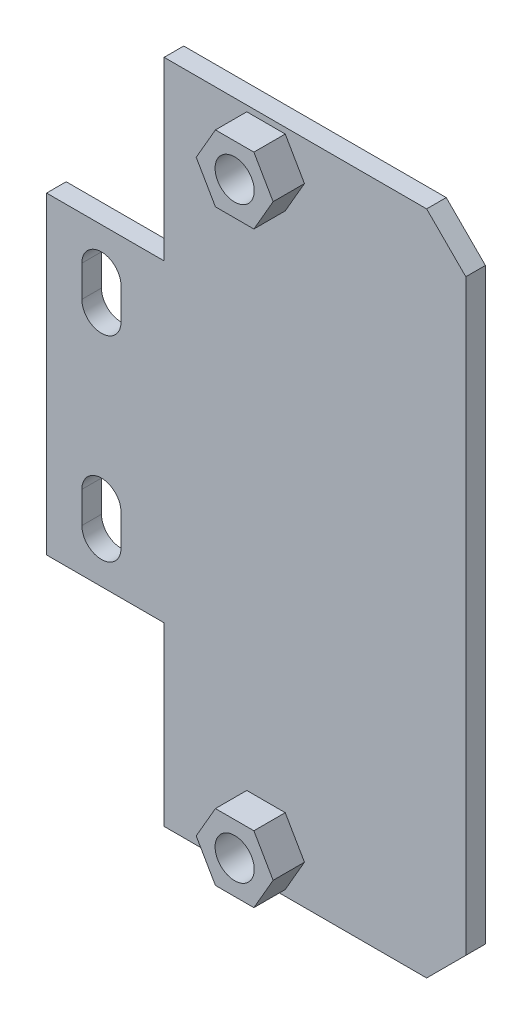
from build123d import *

# Parameters (mm, degrees)
SKETCH_1_W            = 52
SKETCH_1_H            = 170
SKETCH_1_R            = 6.25
EXTRUDE_392_DEPTH     = 5
SKETCH_6_W            = 30
SKETCH_6_H            = 80
EXTRUDE_644_DEPTH     = 5
CUT_EXTRUDE_947_DEPTH = 102.911726509
SKETCH_3_R            = 5
EXTRUDE_2_DEPTH       = 8
EXTRUDE_2_2_DEPTH     = 8
SKETCH_11_W           = 25
SKETCH_11_H           = 170
EXTRUDE_3_DEPTH       = 5
CHAMFER_6_SIZE        = 10


with BuildPart() as part:
    # 草图1 → Extrude 392 (new body)
    with BuildSketch(Plane.XY):
        Rectangle(SKETCH_1_W, SKETCH_1_H)
        with Locations((0, 75)):
            Circle(SKETCH_1_R, mode=Mode.SUBTRACT)
        with Locations((0, -75)):
            Circle(SKETCH_1_R, mode=Mode.SUBTRACT)
    extrude(amount=EXTRUDE_392_DEPTH)

    # 草图6 → Extrude 644 (add)
    with BuildSketch(Plane(origin=(0, 0, 0), x_dir=(-1, 0, 0), z_dir=(0, 0, -1))):
        with Locations((41, 0)):
            Rectangle(SKETCH_6_W, SKETCH_6_H)
    extrude(amount=-EXTRUDE_644_DEPTH)

    # 草图10 → Cut-Extrude 947 (cut, through all)
    with BuildSketch(Plane.XY.offset(5)):
        with BuildLine():
            Line((-47, -29), (-47, -21))
            ThreePointArc((-47, -21), (-42, -16), (-37, -21))
            Line((-37, -21), (-37, -29))
            ThreePointArc((-37, -29), (-42, -34), (-47, -29))
        make_face()
        with BuildLine():
            Line((-47, 29), (-47, 21))
            ThreePointArc((-47, 21), (-42, 16), (-37, 21))
            Line((-37, 21), (-37, 29))
            ThreePointArc((-37, 29), (-42, 34), (-47, 29))
        make_face()
    extrude(amount=-CUT_EXTRUDE_947_DEPTH, mode=Mode.SUBTRACT)


with BuildPart() as body_2:
    # 草图3 → 凸台-拉伸2 (new body)
    with BuildSketch(Plane.XY.offset(5)):
        Polygon((9.814954576, 75), (4.907477288, 83.5), (-4.907477288, 83.5), (-9.814954576, 75), (-4.907477288, 66.5), (4.907477288, 66.5), align=None)
        with Locations((0, 75)):
            Circle(SKETCH_3_R, mode=Mode.SUBTRACT)
    extrude(amount=EXTRUDE_2_DEPTH)


with BuildPart() as body_3:
    # 草图3 → Extrude 2 2 (new body)
    with BuildSketch(Plane.XY.offset(5)):
        Polygon((9.814954576, -75), (4.907477288, -66.5), (-4.907477288, -66.5), (-9.814954576, -75), (-4.907477288, -83.5), (4.907477288, -83.5), align=None)
        with Locations((0, -75)):
            Circle(SKETCH_3_R, mode=Mode.SUBTRACT)
    extrude(amount=EXTRUDE_2_2_DEPTH)


with BuildPart() as body_4:
    # 草图11 → 凸台-拉伸3 (new body)
    with BuildSketch(Plane.XY.offset(5)):
        with Locations((38.5, 0)):
            Rectangle(SKETCH_11_W, SKETCH_11_H)
    extrude(amount=-EXTRUDE_3_DEPTH)


with BuildPart() as part_1:
    add(part.part)

    # Combine 1: union body 4
    add(body_4.part)

    # 倒角6
    chamfer_6_edges = [part_1.edges().sort_by_distance(p)[0] for p in [
        (51, 85, 2.5),
        (51, -85, 2.5),
    ]]
    chamfer(chamfer_6_edges, length=CHAMFER_6_SIZE)


solid = Compound([body_2.part, body_3.part, part_1.part])
